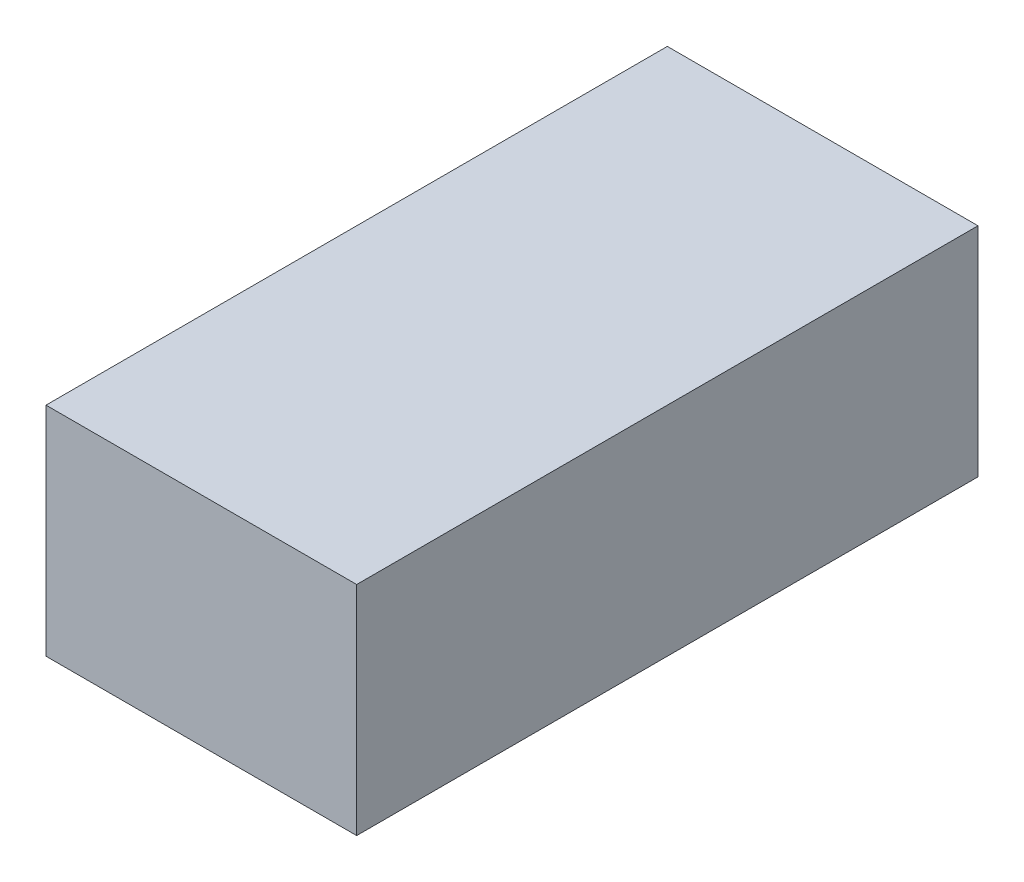
SolidWorks part; units mm, degrees
material "标准件"
ref_plane "前视基准面" through (0, 0, 0) normal (0, 0, 1) x (1, 0, 0)
ref_plane "上视基准面" through (0, 0, 0) normal (0, 1, 0) x (1, 0, 0)
ref_plane "右视基准面" through (0, 0, 0) normal (1, 0, 0) x (0, 0, -1)
sketch "草图1" plane through (0, 0, 0) normal (0, 0, 1) x (1, 0, 0)
  line L1 (-150, 105) -> (150, 105)
  line L2 (-150, 105) -> (-150, -105)
  line L3 (-150, -105) -> (150, -105)
  line L4 (150, 105) -> (150, -105)
  line L5 (-150, 105) -> (150, -105) construction
  line L6 (-150, -105) -> (150, 105) construction
  point P0 (0, 0)
  dimension "D1" = 300
  dimension "D2" = 210
extrude "凸台-拉伸1" add sketch "草图1" along normal blind 600
